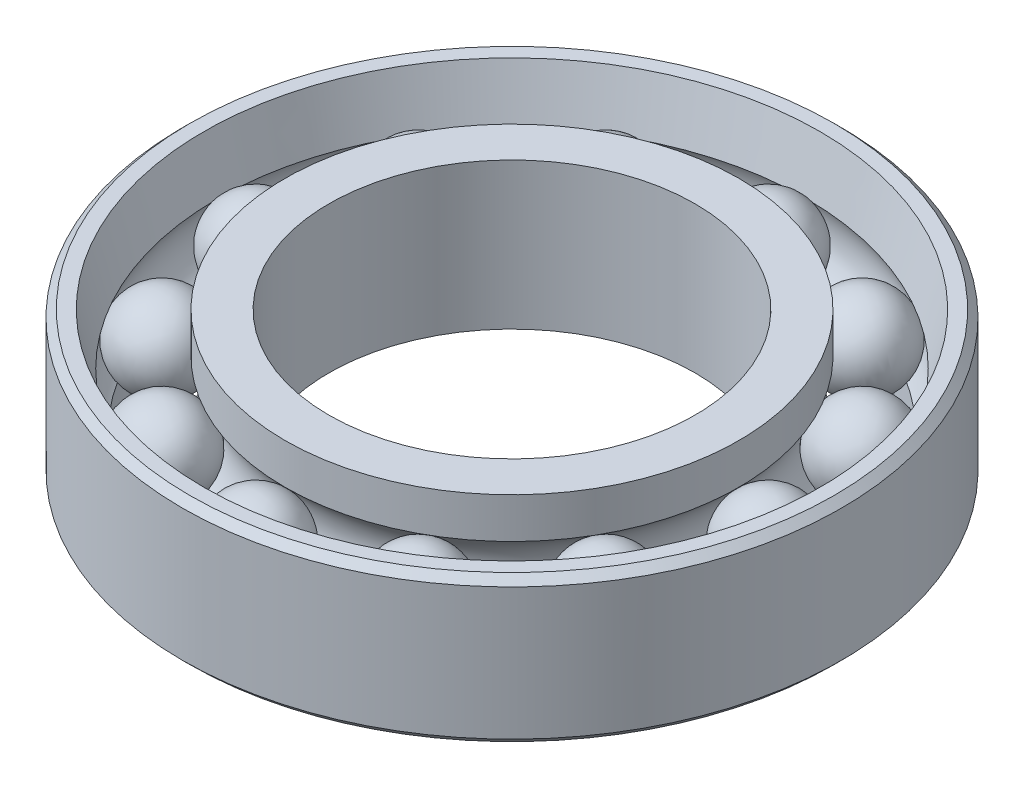
SolidWorks part; units mm, degrees
ref_plane "Front" through (0, 0, 0) normal (0, 0, 1) x (1, 0, 0)
ref_plane "Top" through (0, 0, 0) normal (0, 1, 0) x (1, 0, 0)
ref_plane "Right" through (0, 0, 0) normal (1, 0, 0) x (0, 0, -1)
sketch "Sketch1" plane through (0, 0, 0) normal (0, 0, 1) x (1, 0, 0)
  line L0 (-25, 10) -> (-31, 10)
  line L1 (-40.1962, 3) -> (-67.9397, 19.0177) construction
  line L2 (-45, 10) -> (-45, -10)
  line L3 (-25, 10) -> (-25, -10)
  line L4 (-31, 10) -> (-31, 4.4721)
  line L5 (-31, -4.4721) -> (-31, -10)
  line L6 (-25, -10) -> (-31, -10)
  line L7 (-35, 0) -> (-64.6145, 0) construction
  line L8 (-40.1962, 3) -> (-47.6897, 30.9664) construction
  line L9 (-40.1962, 3) -> (-42.0718, 10)
  line L10 (0, 0) -> (0, -46.601) construction
  line L11 (-39, -4.4721) -> (-39, -10)
  line L12 (-42.0718, 10) -> (-45, 10)
  line L13 (-39, -10) -> (-45, -10)
  arc A0 (-40.1962, 3) -> (-39, -4.4721) centre (-35, 0) ccw
  arc A1 (-31, -4.4721) -> (-31, 4.4721) centre (-35, 0) ccw
  dimension "D1" = 12
  dimension "D3" = 10
  dimension "D8" = 39
  dimension "D2" = 35
  dimension "D4" = 30
  dimension "D5" = 45
  dimension "D6" = 20
  dimension "D7" = 6
  dimension "D9" = 45
revolve "Revolve1" add sketch "Sketch1" angle 360 about L10
sketch "Sketch2" plane through (0, 0, 0) normal (0, 1, 0) x (1, 0, 0)
  line L0 (0, 0) -> (0, 47.8703) construction
  line L1 (0, 29) -> (0, 41)
  arc A0 (0, 29) -> (0, 41) centre (0, 35) ccw
  dimension "D1" = 12
  dimension "D2" = 35
revolve "Revolve2" add sketch "Sketch2" angle 360 about L1
sketch "Sketch3" plane through (0, 0, 0) normal (0, 1, 0) x (1, 0, 0)
  line L0 (0, 0) -> (0, 34.4273) construction
  line L1 (0, 0) -> (-14.1137, 24.4456) construction
  line L2 (-14.5, 25.1147) -> (-20.5, 35.507)
  line L3 (-14.5, 25.1147) -> (-28.2273, 48.8912) construction
  arc A0 (-14.5, 25.1147) -> (-20.5, 35.507) centre (-17.5, 30.3109) ccw
  dimension "D2" = 12
  dimension "D1" = 30
  dimension "D3" = 35
revolve "Revolve3" add sketch "Sketch3" angle 360 about L2
sketch "Sketch4" plane through (0, 0, 0) normal (0, 1, 0) x (1, 0, 0)
  line L0 (0, 0) -> (0, 51.9147) construction
  line L1 (0, 0) -> (-54.6205, 31.5352) construction
  line L2 (-25.1147, 14.5) -> (-35.507, 20.5)
  arc A0 (-25.1147, 14.5) -> (-35.507, 20.5) centre (-30.3109, 17.5) ccw
  dimension "D2" = 12
  dimension "D1" = 60
  dimension "D3" = 35
revolve "Revolve4" add sketch "Sketch4" angle 360 about L2
sketch "Sketch6" plane through (0, 0, 0) normal (0, 1, 0) x (1, 0, 0)
  line L0 (0, 0) -> (0, 51.7338) construction
  line L1 (0, 0) -> (-22.6414, -13.072) construction
  line L2 (-35.507, -20.5) -> (-25.1147, -14.5)
  line L3 (-25.1147, -14.5) -> (-55.3636, -31.9642) construction
  arc A0 (-25.1147, -14.5) -> (-35.507, -20.5) centre (-30.3109, -17.5) ccw
  dimension "D2" = 12
  dimension "D1" = 120
  dimension "D3" = 35
revolve "Revolve6" add sketch "Sketch6" angle 360 about L2
sketch "Sketch7" plane through (0, 0, 0) normal (0, 1, 0) x (1, 0, 0)
  line L0 (0, 0) -> (0, 25) construction
  line L1 (0, 0) -> (-35, -60.6218) construction
  line L2 (-20.5, -35.507) -> (-14.5, -25.1147)
  circle A0 centre (0, 0) radius 25 construction
  arc A1 (-14.5, -25.1147) -> (-20.5, -35.507) centre (-17.5, -30.3109) ccw
  dimension "D2" = 12
  dimension "D1" = 150
  dimension "D3" = 35
revolve "Revolve7" add sketch "Sketch7" angle 360 about L2
sketch "Sketch8" plane through (0, 0, 0) normal (0, 1, 0) x (1, 0, 0)
  line L0 (0, 0) -> (0, -57.9265) construction
  line L1 (0, -29) -> (0, -41)
  arc A0 (0, -29) -> (0, -41) centre (0, -35) ccw
  dimension "D1" = 12
  dimension "D2" = 35
revolve "Revolve8" add sketch "Sketch8" angle 360 about L1
sketch "Sketch9" plane through (0, 0, 0) normal (0, 1, 0) x (1, 0, 0)
  line L0 (0, 0) -> (0, 22.7522) construction
  line L1 (0, 0) -> (25.4595, 44.0971) construction
  line L2 (14.5, 25.1147) -> (20.5, 35.507)
  arc A0 (20.5, 35.507) -> (14.5, 25.1147) centre (17.5, 30.3109) ccw
  dimension "D2" = 12
  dimension "D1" = 30
  dimension "D3" = 35
revolve "Revolve9" add sketch "Sketch9" angle 360 about L2
sketch "Sketch10" plane through (0, 0, 0) normal (0, 1, 0) x (1, 0, 0)
  line L0 (0, 0) -> (0, 64.9432) construction
  line L1 (0, 0) -> (64.6366, 37.318) construction
  line L2 (25.1147, 14.5) -> (35.507, 20.5)
  arc A0 (35.507, 20.5) -> (25.1147, 14.5) centre (30.3109, 17.5) ccw
  dimension "D2" = 12
  dimension "D1" = 60
  dimension "D3" = 35
revolve "Revolve10" add sketch "Sketch10" angle 360 about L2
sketch "Sketch11" plane through (0, 0, 0) normal (0, 1, 0) x (1, 0, 0)
  line L0 (0, 0) -> (0, 58.3052) construction
  line L1 (0, 0) -> (15.4625, 0) construction
  line L2 (29, 0) -> (41, 0)
  line L3 (61.2973, 0) -> (75.3248, 0) construction
  line L4 (29, 0) -> (41, 0) construction
  arc A0 (41, 0) -> (29, 0) centre (35, 0) ccw
  dimension "D2" = 12
  dimension "D1" = 90
  dimension "D3" = 35
revolve "Revolve11" add sketch "Sketch11" angle 360 about L2
sketch "Sketch12" plane through (0, 0, 0) normal (0, 1, 0) x (1, 0, 0)
  line L0 (0, 0) -> (0, 66.8547) construction
  line L1 (25.1147, -14.5) -> (35.507, -20.5)
  arc A0 (35.507, -20.5) -> (25.1147, -14.5) centre (30.3109, -17.5) ccw
  dimension "D2" = 12
  dimension "D3" = 35
revolve "Revolve12" add sketch "Sketch12" angle 360 about L1
sketch "Sketch13" plane through (0, 0, 0) normal (0, 1, 0) x (1, 0, 0)
  line L0 (0, 0) -> (0, 56.5701) construction
  line L1 (0, 0) -> (27.5671, -47.7475) construction
  line L2 (14.5, -25.1147) -> (20.5, -35.507)
  arc A0 (20.5, -35.507) -> (14.5, -25.1147) centre (17.5, -30.3109) ccw
  dimension "D2" = 12
  dimension "D1" = 150
  dimension "D3" = 35
revolve "Revolve13" add sketch "Sketch13" angle 360 about L2
sketch "Sketch14" plane through (0, 0, 0) normal (0, 1, 0) x (1, 0, 0)
  line L0 (0, 0) -> (-66.2251, 0) construction
  line L1 (0, 0) -> (0, 48.3814) construction
  line L2 (-41, 0) -> (-29, 0)
  arc A0 (-29, 0) -> (-41, 0) centre (-35, 0) ccw
  dimension "D1" = 12
  dimension "D2" = 35
revolve "Revolve14" add sketch "Sketch14" angle 360 about L2
chamfer "Chamfer1" distance 1 angle 45 2 edges at (0, 10, 45) (0, -10, 45)
